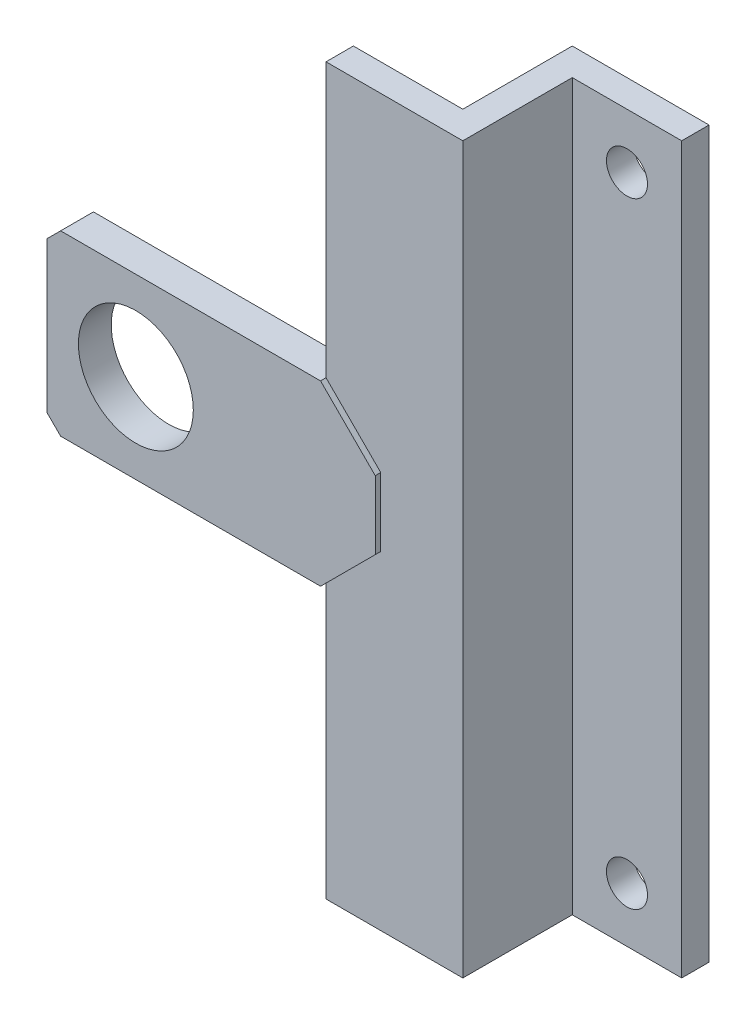
from build123d import *

# Parameters (mm, degrees)
SKETCH_1_R          = 21
EXTRUDE_1_DEPTH     = 12
CHAMFER_1_SIZE      = 5
CHAMFER_2_SIZE      = 20
EXTRUDE_2_DEPTH     = 10
SKETCH_4_W          = 10
SKETCH_4_H          = 265
EXTRUDE_3_DEPTH     = 50
SKETCH_6_W          = 50
SKETCH_6_H          = 265
EXTRUDE_4_DEPTH     = 10
SKETCH_7_R          = 7.5
CUT_EXTRUDE_1_DEPTH = 211.063085762


with BuildPart() as part:
    # 草图1 → 凸台-拉伸1 (new body)
    with BuildSketch(Plane.XY):
        Polygon((32.5, 32.5), (87.5, 32.5), (87.5, -32.5), (32.5, -32.5), (-32.5, -32.5), (-32.5, 32.5), align=None)
        Circle(SKETCH_1_R, mode=Mode.SUBTRACT)
    extrude(amount=EXTRUDE_1_DEPTH)

    # 倒角1
    chamfer_1_edges = [part.edges().sort_by_distance(p)[0] for p in [
        (-32.5, -32.5, 6),
        (-32.5, 32.5, 6),
    ]]
    chamfer(chamfer_1_edges, length=CHAMFER_1_SIZE)

    # 倒角2
    chamfer_2_edges = [part.edges().sort_by_distance(p)[0] for p in [
        (87.5, 32.5, 6),
        (87.5, -32.5, 6),
    ]]
    chamfer(chamfer_2_edges, length=CHAMFER_2_SIZE)

    # 草图3 → 凸台-拉伸2 (add)
    with BuildSketch(Plane(origin=(0, 0, 0), x_dir=(-1, 0, 0), z_dir=(0, 0, -1))):
        Polygon((-67.5, 32.5), (-87.5, 12.5), (-87.5, -12.5), (-67.5, -32.5), (-67.5, -132.5), (-117.5, -132.5), (-117.5, 132.5), (-67.5, 132.5), align=None)
    extrude(amount=-EXTRUDE_2_DEPTH)

    # 草图4 → 凸台-拉伸3 (add)
    with BuildSketch(Plane.XY.offset(10)):
        with Locations((112.5, 0)):
            Rectangle(SKETCH_4_W, SKETCH_4_H)
    extrude(amount=-EXTRUDE_3_DEPTH)

    # 草图6 → 凸台-拉伸4 (add)
    with BuildSketch(Plane(origin=(0, 0, -40), x_dir=(-1, 0, 0), z_dir=(0, 0, -1))):
        with Locations((-132.5, 0)):
            Rectangle(SKETCH_6_W, SKETCH_6_H)
    extrude(amount=-EXTRUDE_4_DEPTH)

    # 草图7 → 切除-拉伸1 (cut, through all)
    with BuildSketch(Plane.XY.offset(-30)):
        with Locations((137.5, 112.5)):
            Circle(SKETCH_7_R)
        with Locations((137.5, -112.5)):
            Circle(SKETCH_7_R)
    extrude(amount=-CUT_EXTRUDE_1_DEPTH, mode=Mode.SUBTRACT)


solid = part.part
